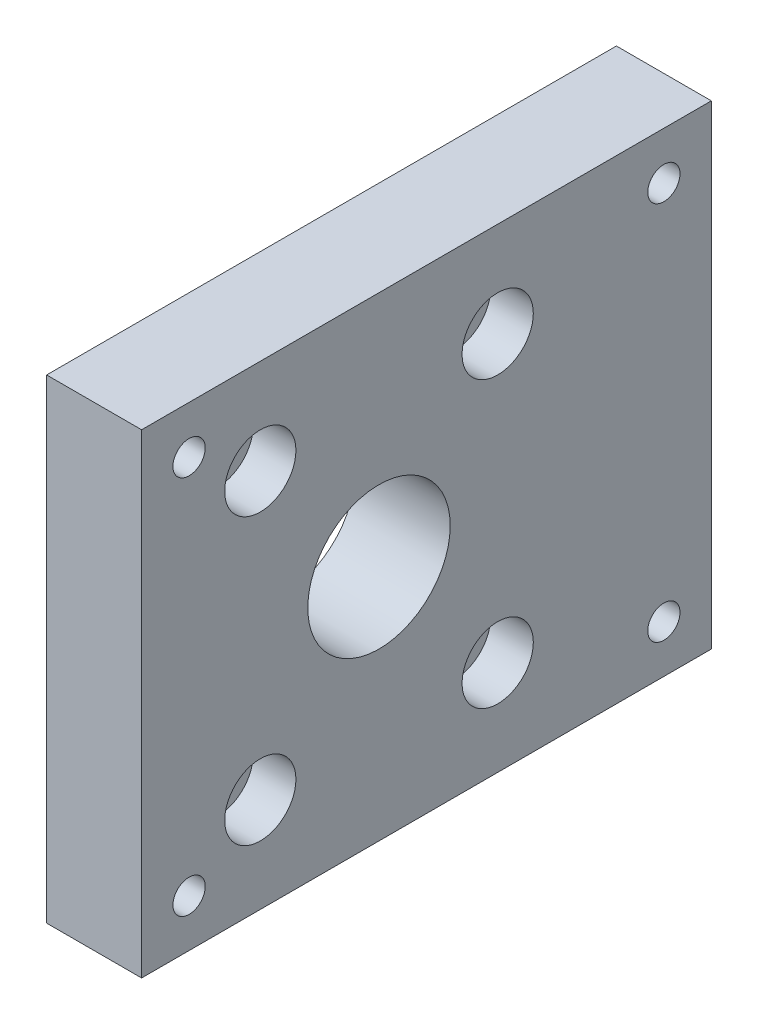
from build123d import *

# Parameters (mm, degrees)
SKETCH_1_W                = 120
SKETCH_1_H                = 100
EXTRUDE_1_DEPTH           = 20
HOLE_WIZARD_1_D           = 9
HOLE_WIZARD_1_CBORE_D     = 15
HOLE_WIZARD_1_CBORE_DEPTH = 9
SKETCH_4_R                = 15
CUT_EXTRUDE_1_DEPTH       = 81.622577483
HOLE_WIZARD_M8_1_D        = 6.8


with BuildPart() as part:
    # 草图1 → 凸台-拉伸1 (new body)
    with BuildSketch(Plane(origin=(0, 0, 0), x_dir=(0, 0, -1), z_dir=(1, 0, 0))):
        Rectangle(SKETCH_1_W, SKETCH_1_H)
    extrude(amount=EXTRUDE_1_DEPTH)

    # 打孔尺寸(%根据)内六角圆柱头螺钉的类型1 (through all)
    with Locations(Plane(origin=(20, 0, 0), x_dir=(0, 0, -1), z_dir=(1, 0, 0))):
        with Locations((-35, 30), (15, 30), (-35, -30), (15, -30)):
            CounterBoreHole(HOLE_WIZARD_1_D / 2, HOLE_WIZARD_1_CBORE_D / 2, HOLE_WIZARD_1_CBORE_DEPTH)

    # 草图4 → 切除-拉伸1 (cut, through all)
    with BuildSketch(Plane(origin=(20, 0, 0), x_dir=(0, 0, -1), z_dir=(1, 0, 0))):
        with Locations((-10, 0)):
            Circle(SKETCH_4_R)
    extrude(amount=-CUT_EXTRUDE_1_DEPTH, mode=Mode.SUBTRACT)

    # M8 螺纹孔1 (through all)
    with Locations(Plane(origin=(20, 0, 0), x_dir=(0, 0, -1), z_dir=(1, 0, 0))):
        with Locations((-50, 40), (-50, -40), (50, -40), (50, 40)):
            Hole(HOLE_WIZARD_M8_1_D / 2)


solid = part.part
